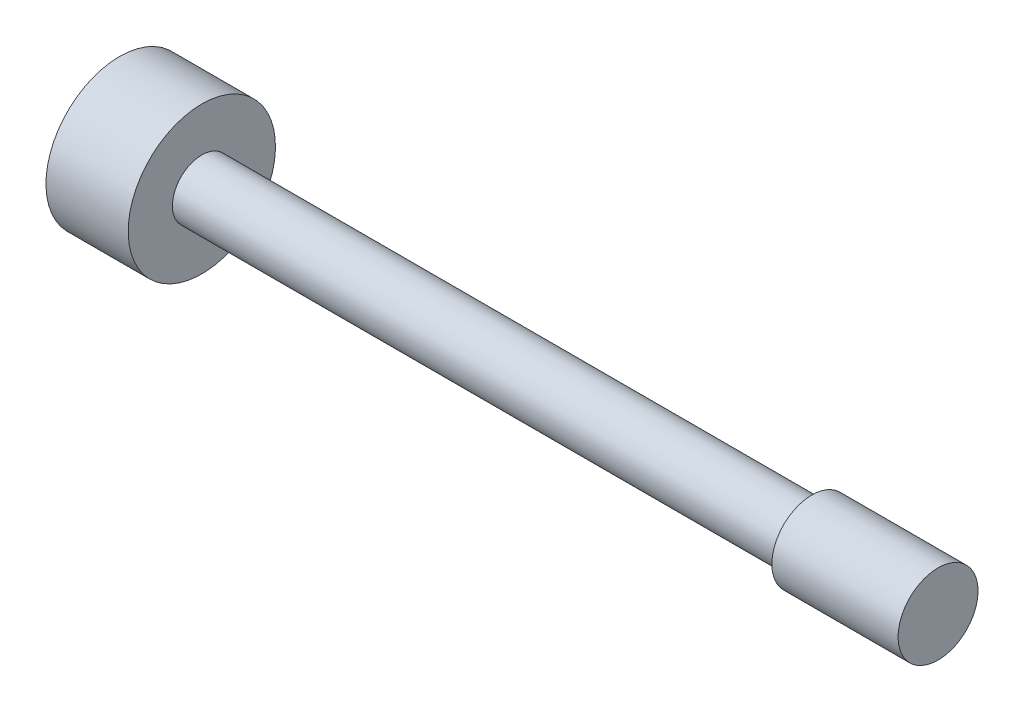
from build123d import *


with BuildPart() as part:
    # Sketch1 → Revolve1 (revolve)
    with BuildSketch(Plane.XY):
        Polygon((0, 0), (0, 3.5), (3.91, 3.5), (3.91, 1.4), (32.91, 1.4), (32.91, 1.9), (38.91, 1.9), (38.91, 0), align=None)
    revolve(axis=Axis((38.91, 0, 0), (-1, 0, 0)))


solid = part.part
